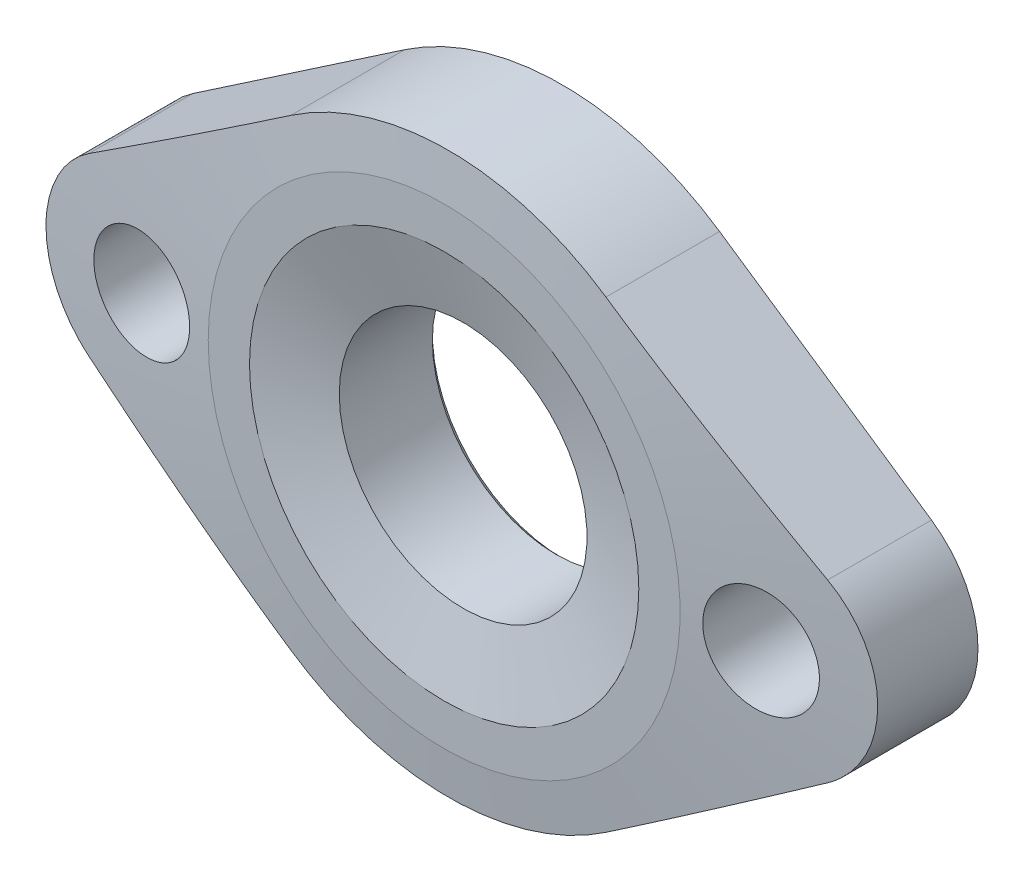
from build123d import *

# Parameters (mm, degrees)
SKETCH1_R           = 9
BOSS_EXTRUDE1_DEPTH = 20
SKETCH5_W           = 21
SKETCH5_H           = 16.784609691
CHAMFER1_SIZE       = 1


with BuildPart() as part:
    # Sketch1 → Boss-Extrude1 (new body)
    with BuildSketch(Plane.XY):
        with BuildLine():
            Line((26.69047619, 39.292091834), (62.614285714, 14.8896348))
            ThreePointArc((62.614285714, 14.8896348), (70.5, 0), (62.614285714, -14.8896348))
            Line((62.614285714, -14.8896348), (26.69047619, -39.292091834))
            ThreePointArc((26.69047619, -39.292091834), (0, -47.5), (-26.69047619, -39.292091834))
            Line((-26.69047619, -39.292091834), (-62.614285714, -14.8896348))
            ThreePointArc((-62.614285714, -14.8896348), (-70.5, 0), (-62.614285714, 14.8896348))
            Line((-62.614285714, 14.8896348), (-26.69047619, 39.292091834))
            ThreePointArc((-26.69047619, 39.292091834), (0, 47.5), (26.69047619, 39.292091834))
        make_face()
        with Locations((52.5, 0)):
            Circle(SKETCH1_R, mode=Mode.SUBTRACT)
        with Locations((-52.5, 0)):
            Circle(SKETCH1_R, mode=Mode.SUBTRACT)
    extrude(amount=BOSS_EXTRUDE1_DEPTH)

    # Sketch5 → Cut-Revolve1 (revolve, cut)
    with BuildSketch(Plane(origin=(0, 0, 0), x_dir=(1, 0, 0), z_dir=(0, 1, 0)), mode=Mode.PRIVATE) as cut_revolve1_sk:
        with Locations((10.5, -8.392304845)):
            Rectangle(SKETCH5_W, SKETCH5_H)
        Polygon((21, -16.784609691), (33, -20), (0, -20), (0, -16.784609691), align=None)
        Polygon((40, -20), (70.5, -20), (70.5, -17), align=None)
    revolve(cut_revolve1_sk.sketch.rotate(Axis((0, 0, 0), (0, 0, 1)), 180), axis=Axis((0, 0, 0), (0, 0, 1)), mode=Mode.SUBTRACT)

    # Chamfer1
    chamfer1_edges = [part.edges().sort_by_distance(p)[0] for p in [
        (21, 0, 0),
    ]]
    chamfer(chamfer1_edges, length=CHAMFER1_SIZE)


solid = part.part
